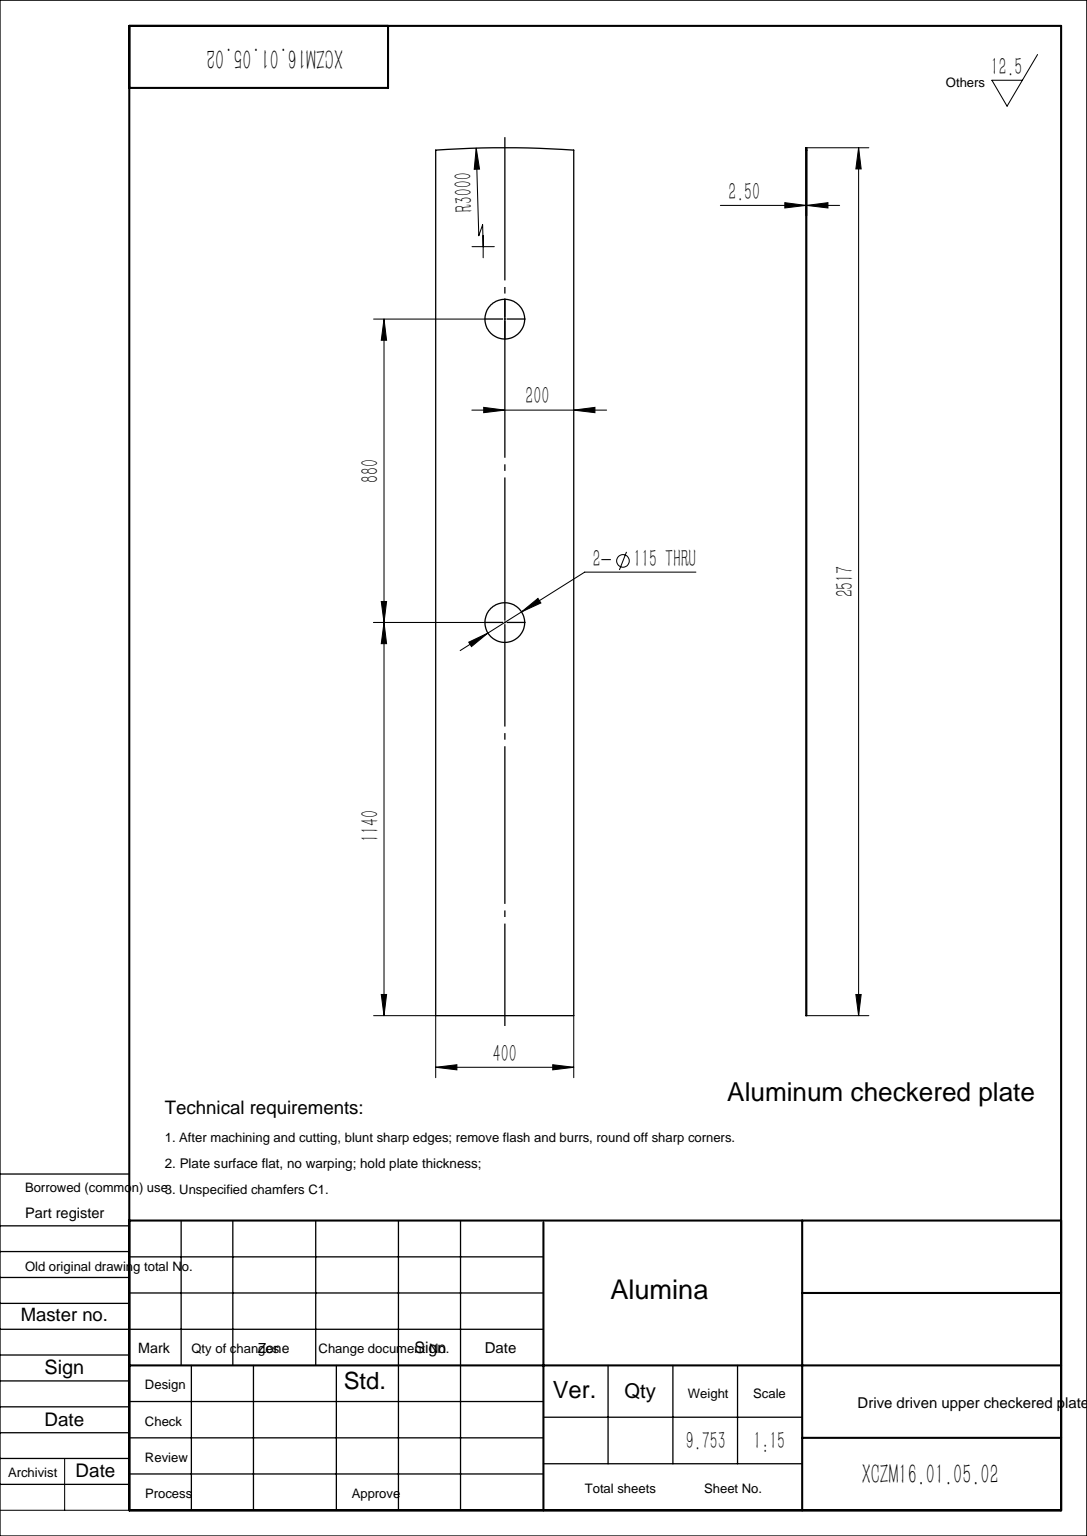
SolidWorks part; units mm, degrees
material "Alumina"
ref_plane "Front Plane" through (0, 0, 0) normal (0, 0, 1) x (1, 0, 0)
ref_plane "Top Plane" through (0, 0, 0) normal (0, 1, 0) x (1, 0, 0)
ref_plane "Right Plane" through (0, 0, 0) normal (1, 0, 0) x (0, 0, -1)
sketch "Sketch1" plane through (0, 0, 0) normal (0, 0, 1) x (1, 0, 0)
  line L0 (-200, 0) -> (200, 0)
  line L1 (200, 0) -> (200, 2510.3259)
  line L2 (0, 0) -> (0, -483) construction
  line L3 (-200, 0) -> (-200, 2510.3259)
  line L4 (0, 0) -> (0, 1140) construction
  line L5 (0, 1140) -> (0, 2020) construction
  arc A0 (200, 2510.3259) -> (-200, 2510.3259) centre (0, -483) ccw
  circle A1 centre (0, 2020) radius 57.5
  circle A2 centre (0, 1140) radius 57.5
  dimension "D1" = 3000
  dimension "D5" = 880
  dimension "D6" = 115
  dimension "D2" = 400
  dimension "D3" = 2517
  dimension "D4" = 1140
extrude "Boss-Extrude1" add sketch "Sketch1" along normal blind 2.5
